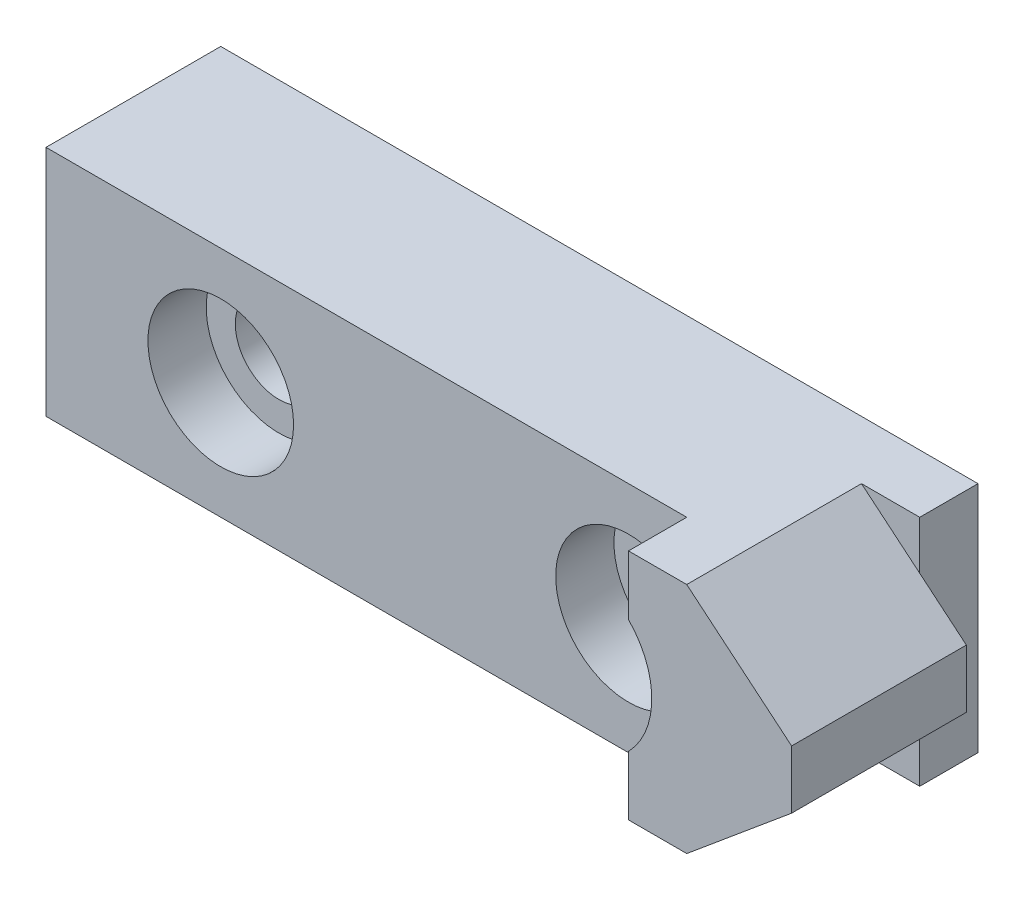
from build123d import *

# Parameters (mm, degrees)
SKETCH1_W           = 130
SKETCH1_H           = 40
BOSS_EXTRUDE1_DEPTH = 10
BOSS_EXTRUDE2_DEPTH = 30
SKETCH3_W           = 110
SKETCH3_H           = 10
CUT_EXTRUDE1_DEPTH  = 40
SKETCH4_R           = 7.5
CUT_EXTRUDE2_DEPTH  = 40
SKETCH5_R           = 14
CUT_EXTRUDE3_DEPTH  = 40
SKETCH6_R           = 12.5
CUT_EXTRUDE4_DEPTH  = 10


with BuildPart() as part:
    # Sketch1 → Boss-Extrude1 (new body)
    with BuildSketch(Plane.XY):
        Rectangle(SKETCH1_W, SKETCH1_H)
    extrude(amount=BOSS_EXTRUDE1_DEPTH)

    # Sketch2 → Boss-Extrude2 (add)
    with BuildSketch(Plane.XY.offset(10)):
        Polygon((-65, 20), (55, 20), (73, 5), (73, -5), (55, -20), (-65, -20), align=None)
    extrude(amount=BOSS_EXTRUDE2_DEPTH)

    # Sketch3 → Cut-Extrude1 (cut)
    with BuildSketch(Plane.XZ.offset(20)):
        with Locations((-10, 35)):
            Rectangle(SKETCH3_W, SKETCH3_H)
    extrude(amount=-CUT_EXTRUDE1_DEPTH, mode=Mode.SUBTRACT)

    # Sketch4 → Cut-Extrude2 (cut)
    with BuildSketch(Plane(origin=(0, 0, 0), x_dir=(-1, 0, 0), z_dir=(0, 0, -1))):
        with Locations((-35, 0)):
            Circle(SKETCH4_R)
        with Locations((35, 0)):
            Circle(SKETCH4_R)
    extrude(amount=-CUT_EXTRUDE2_DEPTH, mode=Mode.SUBTRACT)

    # Sketch5 → Cut-Extrude3 (cut)
    with BuildSketch(Plane.XY.offset(30)):
        with Locations((-35, 0)):
            Circle(SKETCH5_R)
        with Locations((35, 0)):
            Circle(SKETCH5_R)
    extrude(amount=CUT_EXTRUDE3_DEPTH, mode=Mode.SUBTRACT)

    # Sketch6 → Cut-Extrude4 (cut)
    with BuildSketch(Plane.XY.offset(30)):
        with Locations((35, 0)):
            Circle(SKETCH6_R)
        with Locations((-35, 0)):
            Circle(SKETCH6_R)
    extrude(amount=-CUT_EXTRUDE4_DEPTH, mode=Mode.SUBTRACT)


solid = part.part
